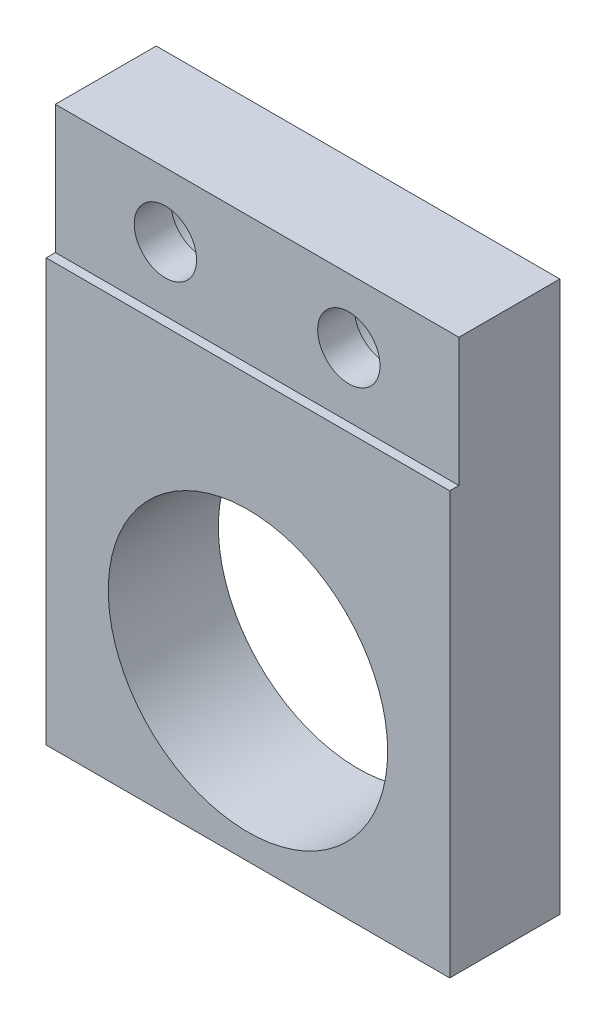
from build123d import *

# Parameters (mm, degrees)
SKETCH_1_W          = 22
SKETCH_1_H          = 30
SKETCH_1_R          = 7.615
SKETCH_1_R_2        = 1.7
EXTRUDE_1_DEPTH     = 6
SKETCH_3_W          = 0.5
SKETCH_3_H          = 7
CUT_EXTRUDE_1_DEPTH = 28.788445632
SKETCH_4_R          = 3
CUT_EXTRUDE_2_DEPTH = 3.5


with BuildPart() as part:
    # 草图1 → 凸台-拉伸1 (new body)
    with BuildSketch(Plane.XY):
        with Locations((-1.935779817, -0.880733945)):
            Rectangle(SKETCH_1_W, SKETCH_1_H)
        with Locations((-1.935779817, -6.880733945)):
            Circle(SKETCH_1_R, mode=Mode.SUBTRACT)
        with Locations((-6.935779817, 10.619266055)):
            Circle(SKETCH_1_R_2, mode=Mode.SUBTRACT)
        with Locations((3.064220183, 10.619266055)):
            Circle(SKETCH_1_R_2, mode=Mode.SUBTRACT)
    extrude(amount=EXTRUDE_1_DEPTH)

    # 草图3 → 切除-拉伸1 (cut, through all)
    with BuildSketch(Plane.ZY.offset(12.935779817)):
        with Locations((5.75, 10.619266055)):
            Rectangle(SKETCH_3_W, SKETCH_3_H)
    extrude(amount=-CUT_EXTRUDE_1_DEPTH, mode=Mode.SUBTRACT)

    # 草图4 → 切除-拉伸2 (cut)
    with BuildSketch(Plane(origin=(0, 0, 0), x_dir=(-1, 0, 0), z_dir=(0, 0, -1))):
        with Locations((-3.064220183, 10.619266055)):
            Circle(SKETCH_4_R)
        with Locations((6.935779817, 10.619266055)):
            Circle(SKETCH_4_R)
    extrude(amount=-CUT_EXTRUDE_2_DEPTH, mode=Mode.SUBTRACT)


solid = part.part
